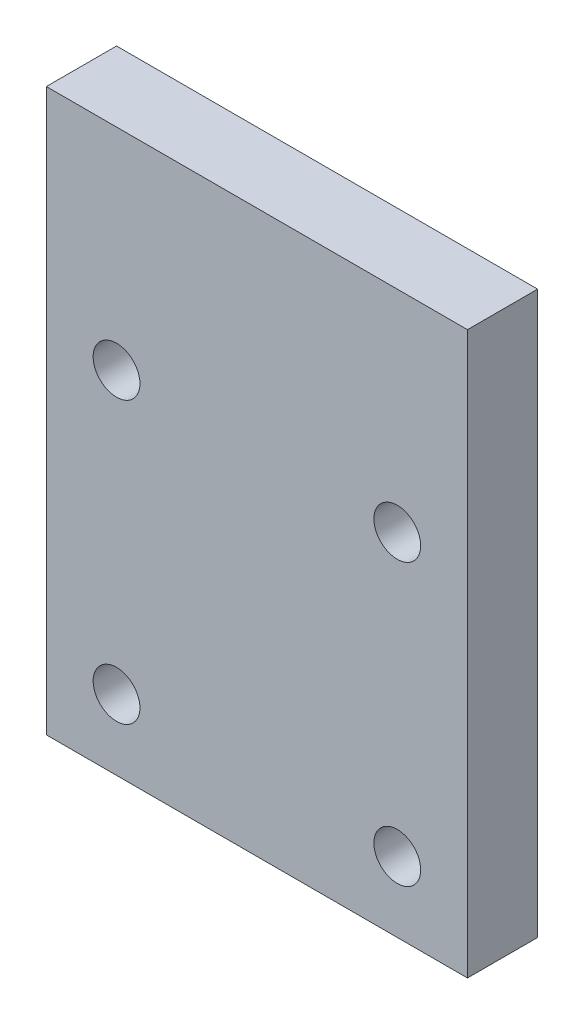
SolidWorks part; units mm, degrees
material "Q235"
ref_plane "Front Plane" through (0, 0, 0) normal (0, 0, 1) x (1, 0, 0)
ref_plane "Top Plane" through (0, 0, 0) normal (0, 1, 0) x (1, 0, 0)
ref_plane "Right Plane" through (0, 0, 0) normal (1, 0, 0) x (0, 0, -1)
sketch "Sketch1" plane through (0, 0, 0) normal (0, 0, 1) x (1, 0, 0)
  line L0 (75, 200) -> (75, 0) construction
  line L1 (0, 0) -> (150, 0)
  line L2 (0, 0) -> (0, 200)
  line L3 (0, 200) -> (150, 200)
  line L4 (150, 0) -> (150, 200)
  dimension "D1" = 150
  dimension "D2" = 200
extrude "Boss-Extrude1" add sketch "Sketch1" along normal blind 25
hole_wizard "3/4-10 Threaded hole1" positions "3DSketch1" profile "Sketch2" tap size "3/4-10" standard "ANSI Inch" end condition through all
sketch3d "3DSketch1"
  line L0 (0, 0, 25) -> (150, 0, 25) construction
  line L1 (150, 0, 25) -> (150, 200, 25) construction
  point P0 (25, 125, 25)
  point P2 (125, 125, 25)
  point P4 (25, 25, 25)
  point P6 (125, 25, 25)
  dimension "D1" = 25
  dimension "D2" = 100
  dimension "D3" = 100
  dimension "D4" = 25
sketch "Sketch2" plane through (25, 125, 25) normal (1, 0, 0) x (0, -1, 0)
  line L0 (0, 0) -> (0, 25)
  line L1 (0, 25) -> (8.3337, 25)
  line L2 (8.3337, 25) -> (8.3337, 0)
  line L5 (8.3337, 0) -> (0, 0)
  line L11 (0, -6.35) -> (0, 107.95) construction
  dimension "通孔螺纹孔钻头直径" = 16.6675
  dimension "通孔螺纹孔钻头深度" = 25
cosmetic thread "孔螺蚊线1"
cosmetic thread "孔螺蚊线2"
cosmetic thread "孔螺蚊线3"
cosmetic thread "孔螺蚊线4"
